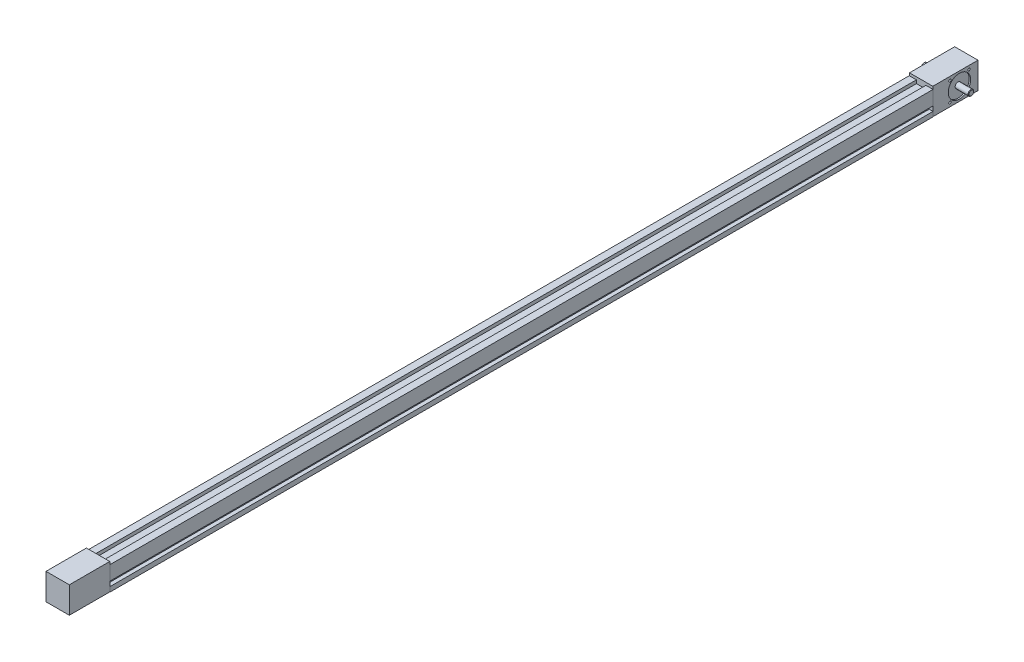
SolidWorks part; units mm, degrees
ref_plane "前视" through (0, 0, 0) normal (0, 0, 1) x (1, 0, 0)
ref_plane "上视" through (0, 0, 0) normal (0, 1, 0) x (1, 0, 0)
ref_plane "右视" through (0, 0, 0) normal (1, 0, 0) x (0, 0, -1)
sketch "草图1" plane through (0, 0, 0) normal (0, 0, 1) x (1, 0, 0)
  line L0 (15, 50) -> (15, 43)
  line L1 (0, 0) -> (50, 0)
  line L2 (0, 0) -> (0, 10)
  line L3 (0, 50) -> (15, 50)
  line L4 (50, 0) -> (50, 10)
  line L5 (15, 43) -> (35, 43)
  line L6 (35, 43) -> (35, 50)
  line L7 (35, 50) -> (50, 50)
  line L8 (0, 20) -> (8, 20)
  line L10 (0, 10) -> (8, 10)
  line L11 (8, 20) -> (8, 10)
  line L12 (50, 20) -> (42, 20)
  line L13 (0, 20) -> (0, 50)
  line L14 (50, 10) -> (42, 10)
  line L15 (42, 20) -> (42, 10)
  line L16 (50, 20) -> (50, 50)
  dimension "D1" = 50
  dimension "D2" = 50
  dimension "D3" = 8
  dimension "D4" = 10
  dimension "D5" = 10
  dimension "D6" = 10
  dimension "D7" = 10
  dimension "D8" = 8
  dimension "D9" = 20
  dimension "D10" = 15
  dimension "D11" = 7
extrude "基体-拉伸" add sketch "草图1" along normal blind 1730
sketch "草图2" plane through (0, 0, 1730) normal (0, 0, 1) x (1, 0, 0)
  line L0 (0, 0) -> (50, 0) construction
  line L1 (0.5, 0) -> (49.5, 0)
  line L2 (0.5, 0) -> (0.5, 55.5)
  line L3 (0.5, 55.5) -> (49.5, 55.5)
  line L4 (49.5, 0) -> (49.5, 55.5)
  line L5 (50, 0) -> (50, 10) construction
  line L6 (0, 10) -> (0, 0) construction
  dimension "D1" = 55.5
  dimension "D2" = 0.5
  dimension "D3" = 0.5
extrude "凸台-拉伸1" add sketch "草图2" along normal blind 85
sketch "草图4" plane through (0, 0, 0) normal (0, 0, -1) x (-1, 0, 0)
  line L0 (-49.5, 50) -> (-49.5, 55.5) construction
  line L1 (-0.5, 0) -> (-49.5, 0)
  line L2 (-0.5, 0) -> (-0.5, 55.5)
  line L3 (-0.5, 55.5) -> (-49.5, 55.5)
  line L4 (-49.5, 0) -> (-49.5, 55.5)
  line L5 (-49.5, 55.5) -> (-0.5, 55.5) construction
  line L6 (-0.5, 55.5) -> (-0.5, 50) construction
extrude "凸台-拉伸3" add sketch "草图4" along normal blind 95
sketch "草图9" plane through (49.5, 0, 0) normal (1, 0, 0) x (0, 0, -1)
  line L0 (-1815, 0) -> (95, 0) construction
  line L3 (95, 55.5) -> (95, 0) construction
  circle A0 centre (56, 27.75) radius 23.5
  dimension "D3" = 47
  dimension "D1" = 39
  dimension "D2" = 27.75
extrude "切除-拉伸5" cut sketch "草图9" against normal blind 3
sketch "草图10" plane through (46.5, 0, 0) normal (1, 0, 0) x (0, 0, -1)
  circle A0 centre (56, 27.75) radius 6
  dimension "D1" = 12
extrude "凸台-拉伸4" add sketch "草图10" along normal blind 28
chamfer "倒角1" distance 1 angle 45 1 edges at (74.5, 27.75, -62)
sketch "草图11" plane through (50, 0, 0) normal (1, 0, 0) x (0, 0, -1)
  line L0 (76, 47.75) -> (56, 27.75) construction
  line L1 (56, 27.75) -> (54.0318, 27.75) construction
  circle A0 centre (56, 27.75) radius 23.5 construction
  point P0 (76, 47.75)
  dimension "D1" = 45
  dimension "D2" = 20
hole_wizard "M5 螺纹孔1" positions "3D草图1" profile "草图12" tap size "M5" standard "GB"
sketch3d "3D草图1"
  point P0 (50, 47.75, -76)
sketch "草图12" plane through (50, 47.75, -76) normal (0, 1, 0) x (0, 0, -1)
  line L0 (0, 0) -> (0, 15.2618)
  line L1 (0, 15.2618) -> (2.1, 14)
  line L2 (2.1, 14) -> (2.1, 10)
  line L3 (2.1, 10) -> (2.5, 10)
  line L4 (2.5, 10) -> (2.5, 0)
  line L5 (2.5, 0) -> (0, 0)
  line L10 (0, 15.2618) -> (-2.1, 14) construction
  line L11 (0, -6.35) -> (0, 107.95) construction
  dimension "螺纹孔钻头直径" = 4.2
  dimension "螺纹孔钻头深度" = 14
  dimension "螺纹主直径" = 5
  dimension "螺纹深度" = 10
  dimension "导头角度" = 118
pattern_circular "阵列(圆周)1" count 4 over 360 about axis through (0, 27.75, -56) along (1, 0, 0) of "M5 螺纹孔1"
ref_plane "基准面1" through (25, 0, 0) normal (1, 0, 0) x (0, 0, -1)
mirror "镜向1" about plane through (25, 0, 0) normal (1, 0, 0) of "阵列(圆周)1", "M5 螺纹孔1", "凸台-拉伸4", "切除-拉伸5"
